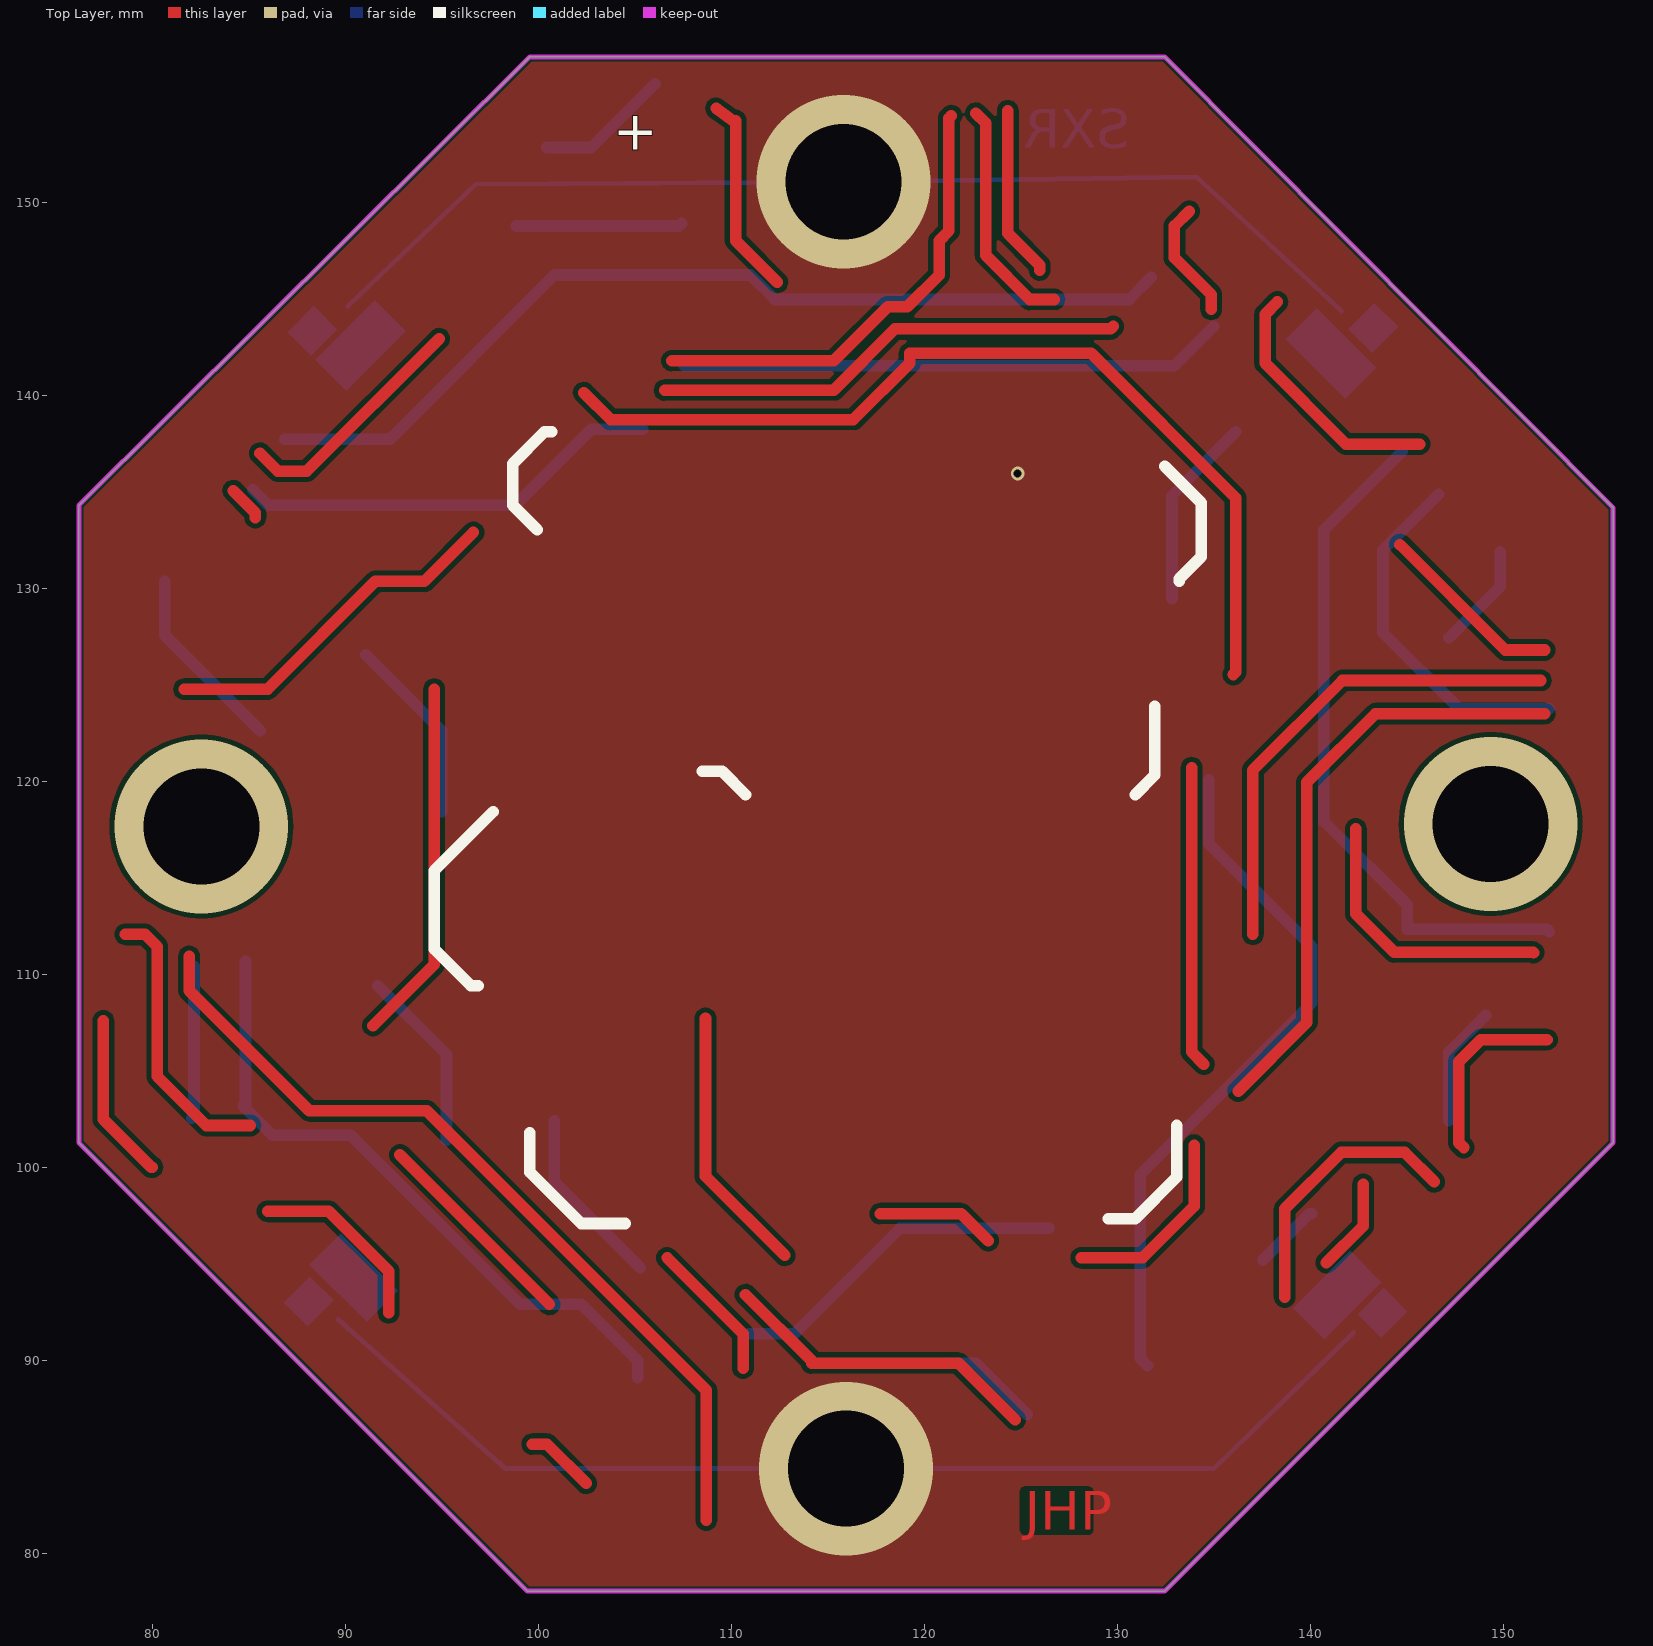
[diagram p0: Top Layer view]
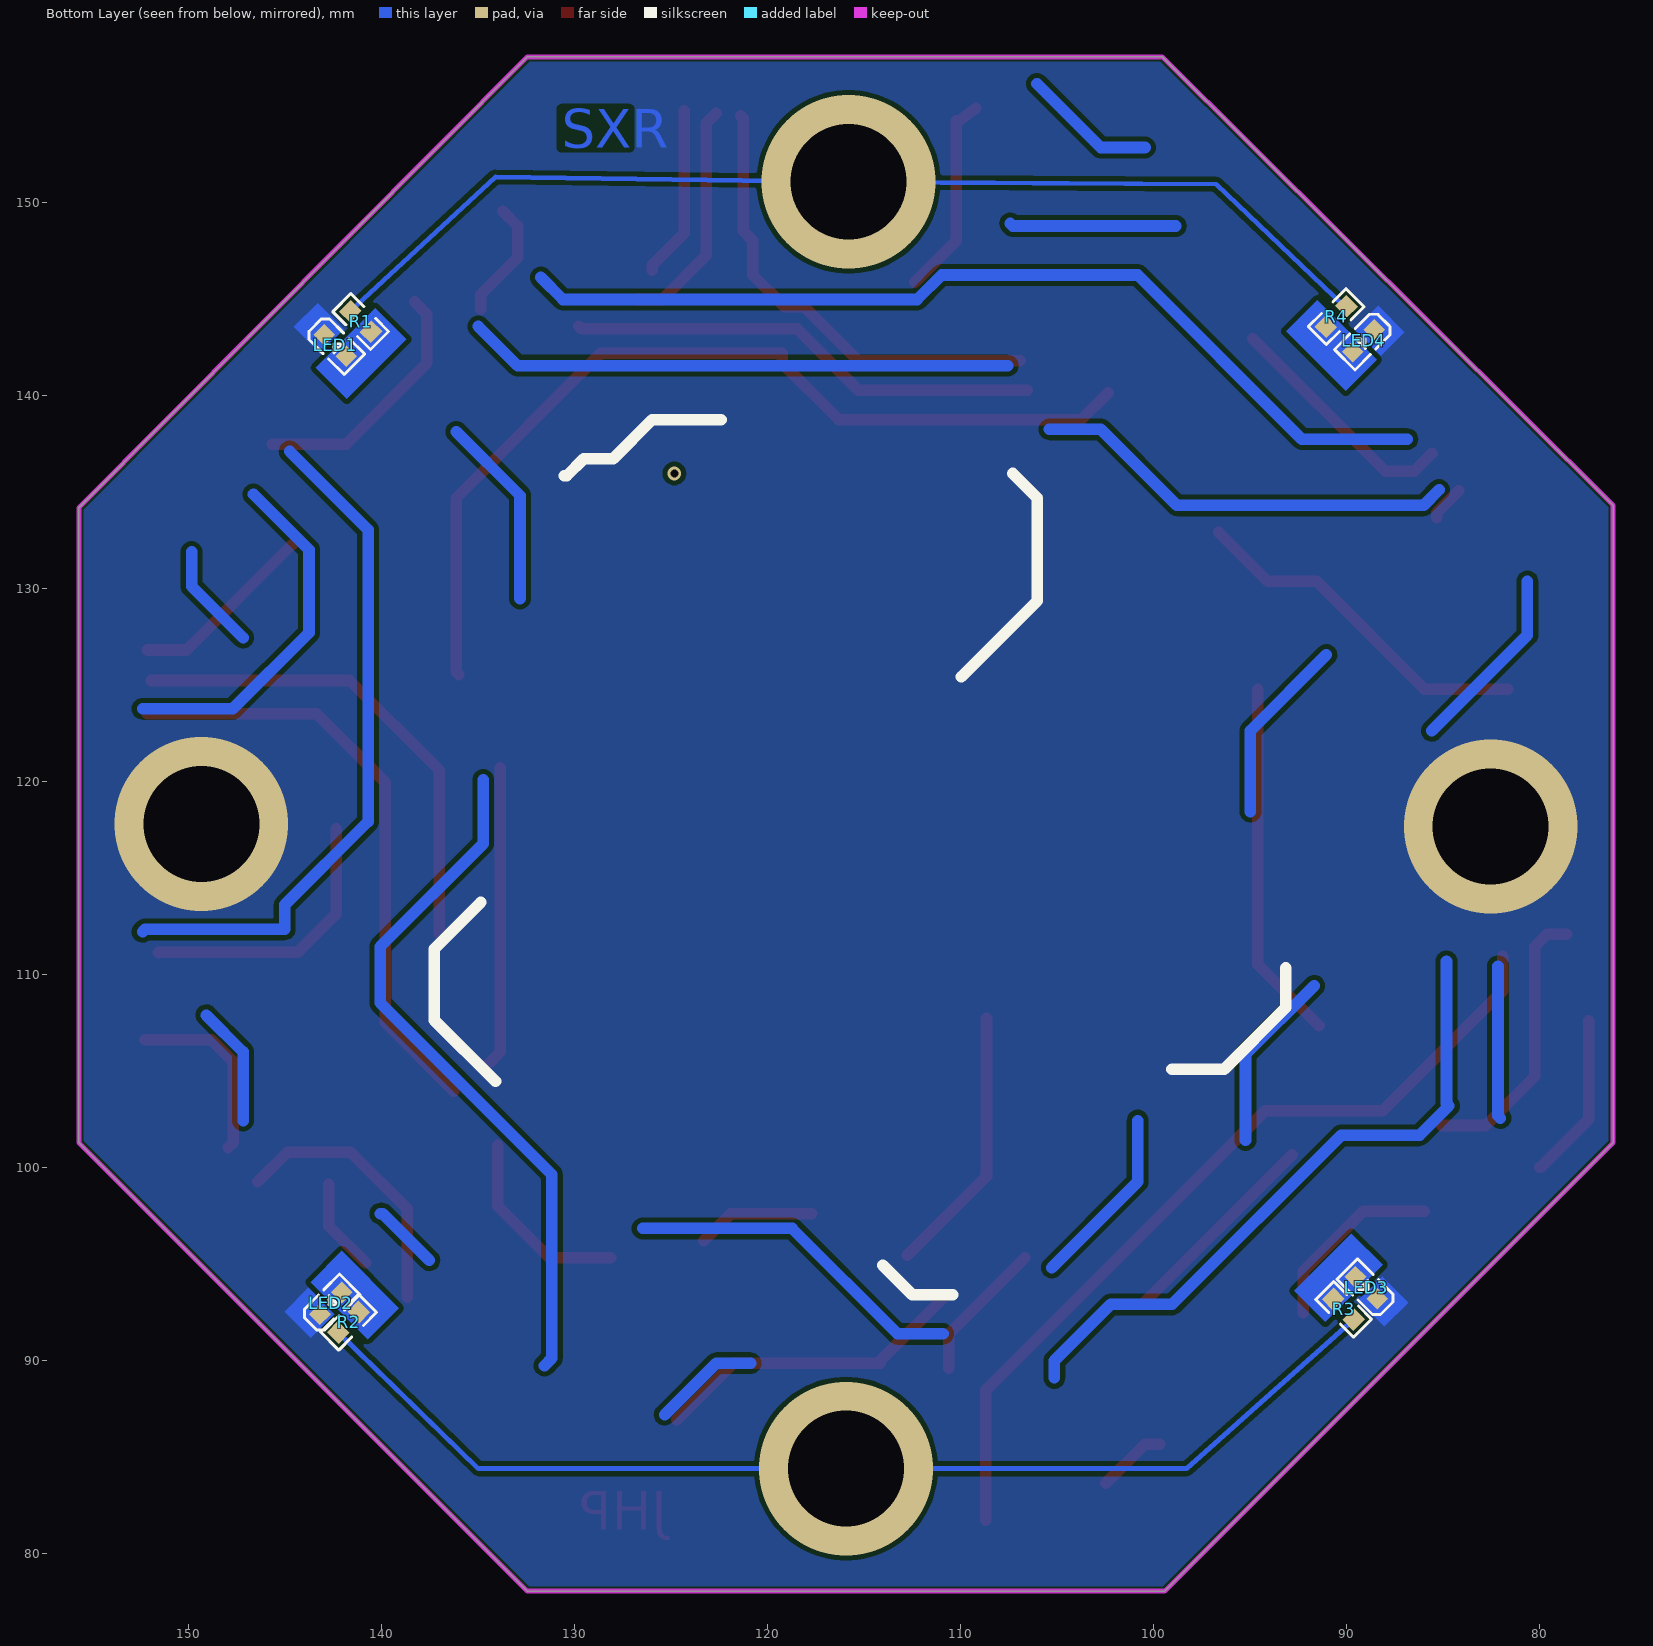
[diagram p1: Bottom Layer view, seen from below]
# Altium PCB MISC51832.pcbdoc
Units mm, origin at the board's own origin, x right, y up, seen from the top; angles counter-clockwise.
Board outline 79.5 x 79.5 mm, 2 copper layers (Top Layer, Bottom Layer), stack 1.58 mm thick; 8 components, 6 nets, 16 pads, 5 vias.

## Layer stack, top to bottom
Top Solder Mask Layer: solder mask 0.01, Dk 3.3
Top Layer: signal copper 0.035
Dielectric1: surface 1.51, FR4, Dk 4.5
Bottom Layer: signal copper 0.035
Bottom Solder Mask Layer: solder mask 0.01, Dk 3.3

## Board outline
76.2,101.265 99.441,78.024 132.461,78.024 155.702,101.265 155.702,134.158 132.461,157.526 99.568,157.526 76.2,134.285

## Design rules (kind name [scope] priority, off if disabled: settings)
BoardOutlineClearance copperThickness2oz_1 [All] p2 off: genericclearance=0.203 ignorepadtopadclearanceinfootprint=FALSE except(0: Arc-SplitContinuation Track-SplitContinuation SMDPad-SplitContinuation THPad-SplitContinuation Via-SplitContinuation Fill-SplitContinuation Region-SplitContinuation Poly-SplitContinuation Text-SplitContinuation Hole-SplitContinuation; 0.152: Arc-CutoutEdge Track-CutoutEdge SMDPad-CutoutEdge THPad-CutoutEdge Via-CutoutEdge Text-CutoutEdge; 0.175: Hole-OutlineEdge Hole-CutoutEdge; 0.254: Poly-OutlineEdge Poly-CutoutEdge; 0.3: Arc-OutlineEdge Track-OutlineEdge SMDPad-OutlineEdge THPad-OutlineEdge Via-OutlineEdge Fill-OutlineEdge Region-OutlineEdge Text-OutlineEdge Fill-CutoutEdge Region-CutoutEdge)
BoardOutlineClearance Plane_innerPlane_1 [All] p4 off: genericclearance=0.102 ignorepadtopadclearanceinfootprint=FALSE except(0: Arc-SplitContinuation Track-SplitContinuation SMDPad-SplitContinuation THPad-SplitContinuation Via-SplitContinuation Fill-SplitContinuation Region-SplitContinuation Poly-SplitContinuation Text-SplitContinuation Hole-SplitContinuation; 0.152: Arc-CutoutEdge Track-CutoutEdge SMDPad-CutoutEdge THPad-CutoutEdge Via-CutoutEdge Text-CutoutEdge; 0.175: Hole-OutlineEdge Hole-CutoutEdge; 0.254: Poly-OutlineEdge Poly-CutoutEdge; 0.3: Arc-OutlineEdge Track-OutlineEdge SMDPad-OutlineEdge THPad-OutlineEdge Via-OutlineEdge Fill-OutlineEdge Region-OutlineEdge Text-OutlineEdge Fill-CutoutEdge Region-CutoutEdge)
BoardOutlineClearance Copper_copperRegion_1 [All] p6 off: genericclearance=0.102 ignorepadtopadclearanceinfootprint=FALSE except(0: Arc-SplitContinuation Track-SplitContinuation SMDPad-SplitContinuation THPad-SplitContinuation Via-SplitContinuation Fill-SplitContinuation Region-SplitContinuation Poly-SplitContinuation Text-SplitContinuation Hole-SplitContinuation; 0.152: Arc-CutoutEdge Track-CutoutEdge SMDPad-CutoutEdge THPad-CutoutEdge Via-CutoutEdge Text-CutoutEdge; 0.175: Hole-OutlineEdge Hole-CutoutEdge; 0.254: Poly-OutlineEdge Poly-CutoutEdge; 0.3: Arc-OutlineEdge Track-OutlineEdge SMDPad-OutlineEdge THPad-OutlineEdge Via-OutlineEdge Fill-OutlineEdge Region-OutlineEdge Text-OutlineEdge Fill-CutoutEdge Region-CutoutEdge)
BoardOutlineClearance copperThickness1oz_1 [All] p8: genericclearance=0.102 ignorepadtopadclearanceinfootprint=FALSE except(0: Arc-SplitContinuation Track-SplitContinuation SMDPad-SplitContinuation THPad-SplitContinuation Via-SplitContinuation Fill-SplitContinuation Region-SplitContinuation Poly-SplitContinuation Text-SplitContinuation Hole-SplitContinuation; 0.152: Arc-CutoutEdge Track-CutoutEdge SMDPad-CutoutEdge THPad-CutoutEdge Via-CutoutEdge Text-CutoutEdge; 0.175: Hole-OutlineEdge Hole-CutoutEdge; 0.254: Poly-OutlineEdge Poly-CutoutEdge; 0.3: Arc-OutlineEdge Track-OutlineEdge SMDPad-OutlineEdge THPad-OutlineEdge Via-OutlineEdge Fill-OutlineEdge Region-OutlineEdge Text-OutlineEdge Fill-CutoutEdge Region-CutoutEdge)
Clearance copperThickness2oz [All] p1 off: gap=0.203 ignorepadtopadclearanceinfootprint=FALSE except(0.152: SMDPad-Track SMDPad-SMDPad THPad-Track SMDPad-THPad THPad-THPad Track-Via SMDPad-Via THPad-Via Via-Via Fill-SMDPad Region-SMDPad Fill-THPad Region-THPad Fill-Via Region-Via Fill-Fill Fill-Region Region-Region Arc-Track Arc-SMDPad Arc-THPad Arc-Via Fill-Arc Region-Arc Arc-Arc Text-Track SMDPad-Text Text-THPad Text-Via Fill-Text Region-Text Arc-Text Text-Text; 0.175: Hole-Track Hole-SMDPad Hole-THPad Hole-Via Fill-Hole Region-Hole Hole-Arc Hole-Text; 0.254: Poly-Track Poly-SMDPad Poly-THPad Poly-Via Poly-Fill Poly-Region Poly-Poly Poly-Arc Poly-Text Poly-Hole; 0.3: Fill-Track Region-Track)
Clearance Plane_innerPlane [All] p3 off: gap=0.102 ignorepadtopadclearanceinfootprint=FALSE except(0.152: SMDPad-Track SMDPad-SMDPad THPad-Track SMDPad-THPad THPad-THPad Track-Via SMDPad-Via THPad-Via Via-Via Fill-SMDPad Region-SMDPad Fill-THPad Region-THPad Fill-Via Region-Via Fill-Fill Fill-Region Region-Region Arc-Track Arc-SMDPad Arc-THPad Arc-Via Fill-Arc Region-Arc Arc-Arc Text-Track SMDPad-Text Text-THPad Text-Via Fill-Text Region-Text Arc-Text Text-Text; 0.175: Hole-Track Hole-SMDPad Hole-THPad Hole-Via Fill-Hole Region-Hole Hole-Arc Hole-Text; 0.254: Poly-Track Poly-SMDPad Poly-THPad Poly-Via Poly-Fill Poly-Region Poly-Poly Poly-Arc Poly-Text Poly-Hole; 0.3: Fill-Track Region-Track)
Clearance Copper_copperRegion [All] p5 off: gap=0.102 ignorepadtopadclearanceinfootprint=FALSE except(0.152: SMDPad-Track SMDPad-SMDPad THPad-Track SMDPad-THPad THPad-THPad Track-Via SMDPad-Via THPad-Via Via-Via Fill-SMDPad Region-SMDPad Fill-THPad Region-THPad Fill-Via Region-Via Fill-Fill Fill-Region Region-Region Arc-Track Arc-SMDPad Arc-THPad Arc-Via Fill-Arc Region-Arc Arc-Arc Text-Track SMDPad-Text Text-THPad Text-Via Fill-Text Region-Text Arc-Text Text-Text; 0.175: Hole-Track Hole-SMDPad Hole-THPad Hole-Via Fill-Hole Region-Hole Hole-Arc Hole-Text; 0.254: Poly-Track Poly-SMDPad Poly-THPad Poly-Via Poly-Fill Poly-Region Poly-Poly Poly-Arc Poly-Text Poly-Hole; 0.3: Fill-Track Region-Track)
Clearance copperThickness1oz [All] p7: gap=0.102 ignorepadtopadclearanceinfootprint=FALSE except(0.152: SMDPad-Track SMDPad-SMDPad THPad-Track SMDPad-THPad THPad-THPad Track-Via SMDPad-Via THPad-Via Via-Via Fill-SMDPad Region-SMDPad Fill-THPad Region-THPad Fill-Via Region-Via Fill-Fill Fill-Region Region-Region Arc-Track Arc-SMDPad Arc-THPad Arc-Via Fill-Arc Region-Arc Arc-Arc Text-Track SMDPad-Text Text-THPad Text-Via Fill-Text Region-Text Arc-Text Text-Text; 0.175: Hole-Track Hole-SMDPad Hole-THPad Hole-Via Fill-Hole Region-Hole Hole-Arc Hole-Text; 0.254: Poly-Track Poly-SMDPad Poly-THPad Poly-Via Poly-Fill Poly-Region Poly-Poly Poly-Arc Poly-Text Poly-Hole; 0.3: Fill-Track Region-Track)
DiffPairsRouting differentialPair [All] p1: maxlimit=0.152 minlimit=0.152 mostfreqgap=0.152 toplayer_minwidth=0.127 toplayer_prefwidth=0.254 toplayer_maxwidth=2.54 toplayer_mingap=0.152 toplayer_prefgap=0.152 toplayer_maxgap=0.152 bottomlayer_minwidth=0.127 bottomlayer_prefwidth=0.254 bottomlayer_maxwidth=2.54 bottomlayer_mingap=0.152 bottomlayer_prefgap=0.152 bottomlayer_maxgap=0.152 maxuncoupledlength=0.254
HoleToHoleClearance otherClearance [All] p1: gap=0.3 allowstackedmicrovias=TRUE
Length netLength [All] p1: minlimit=0 maxlimit=0
PasteMaskExpansion pasteMaskExpansion [All] p1: expansion=0
PlaneConnect innerPlane [All] p1: planeconnectstyle=Relief reliefexpansion=0.508 reliefentries=4 reliefconductorwidth=0.254 reliefairgap=0.254
PolygonConnect copperRegion [All] p1: connectstyle=Relief reliefconductorwidth=0.254 reliefentries=4 polygonreliefangle="90 Angle" airgapwidth=0.254 via.connectstyle=Relief via.reliefconductorwidth=0.254 via.reliefentries=4 via.polygonreliefangle="90 Angle" via.airgapwidth=0.254
RoutingVias viaSize [All] p1: holewidth=0.305 width=0.61 viastyle="Through Hole" minholewidth=0.3 minwidth=0.5 maxholewidth=6.3 maxwidth=10
SolderMaskExpansion solderMaskExpansion [IsVia] p1: expansion=-25.4 istentingtop=TRUE
SolderMaskExpansion solderMaskExpansion [All] p2: expansion=0.051 istentingtop=FALSE
Width copperThickness2oz_2 [All] p1 off: maxlimit=2.54 minlimit=0.203 preferedwidth=0.254
Width copperThickness1oz_2 [All] p2: maxlimit=2.54 minlimit=0.127 preferedwidth=0.254

## Components (designator, comment, footprint, x,y, rotation, side; value= is the part's Value field where it differs from the comment)
LED1 "" LED_0603 142.367,142.54 r225 bottom
LED2 "" LED_0603 142.614,92.975 r135 bottom
LED3 "" LED_0603 89.027,93.772 r45 bottom
LED4 "" LED_0603 89.165,142.776 r315 bottom
R1 "3.3k" R0603 141.097,143.81 r225 bottom
R2 "3.3k" R0603 141.725,91.959 r135 bottom
R3 "3.3k" R0603 90.17,92.629 r45 bottom
R4 "3.3k" R0603 90.551,144.064 r315 bottom

## Footprints (in the part's own frame and the unit in brackets; to place one, negate y for a bottom-side part, rotate by r counter-clockwise, add the part's x,y. Pads: shape width x height; smd on the part's side, far side on the other; paste and mask are expansions set on the pad)
LED_0603 [mil]
  rect 31.5x31.5 smd paste+0 mask+2: 1(-33.5,-0.4) 2(29.5,-0.2)
  silkscreen extent -61,-30 53,29
R0603 [mm]
  rect 0.806x0.864 smd paste-100 mask+0.051: 1(-0.753,0) 2(0.753,0)
  silkscreen extent -1.39,-0.66 1.39,0.66

## Via types
v1: diameter 9, hole 5.999, Top Layer to Bottom Layer, 4 vias
v2: diameter 0.7, hole 0.399, Top Layer to Bottom Layer, 1 vias

## Nets (pads, with @x,y where several pads share a name; then routed paths per layer and width w, separated by ;. In a path a pad name is that pad's centre, name@x,y a point inside that pad or via, vN(x,y) a via of type N, cw(c..) or ccw(c..) an arc to the next point about the centre after c; other vN are vias at no path point)
$1N377: LED1.2 R1.2
$1N381: LED2.2 R2.2
$1N385: LED3.2 R3.2
$1N390: LED4.2 R4.2
+5V: R1.1 R2.1 R3.1 R4.1 | length 450.8
  Bottom Layer w0.254: R3.1 98.298,84.374 v1(115.951,84.374) 135.001,84.374 R2.1 ; R4.1@90.145,144.597 96.774,150.922 v1(115.824,151.049) 134.112,151.303 R1.1
  Bottom Layer w0.6: 80.645,130.348 80.645,127.554 85.598,122.601 ; 82.042,102.535 82.169,102.662 82.169,110.409 ; 84.836,110.663 84.836,103.297 84.709,103.17 86.233,101.646 90.297,101.646 99.06,92.883 102.235,92.883 105.156,89.962 105.156,89.073 ; 85.222,135.086 86.024,134.285 98.806,134.285 102.743,138.222 105.41,138.222 ; 86.868,137.714 92.329,137.714 100.838,146.223 110.998,146.223 112.268,144.953 130.617,144.953 131.76,146.096 ; 91.059,126.538 94.996,122.601 94.996,118.41 ; 91.694,109.393 95.25,105.837 95.25,101.392 ; 98.859,148.761 107.313,148.761 107.442,148.89 ; 100.457,152.827 102.751,152.827 106.053,156.129 ; 100.838,102.408 100.838,99.233 105.283,94.788 ; 107.569,141.524 132.969,141.524 135.001,143.556 ; 110.924,91.359 113.284,91.359 118.745,96.82 126.492,96.82 ; 120.896,89.835 122.682,89.835 125.349,87.168 ; 131.572,89.708 131.191,90.089 131.191,99.614 140.081,108.504 140.081,111.425 134.747,116.759 134.747,120.061 ; 132.842,129.459 132.842,134.793 136.144,138.095 ; 137.541,95.169 139.954,97.582 140.081,97.582 ; 144.78,137.079 140.716,133.015 140.716,117.902 145.034,113.584 145.034,112.314 152.273,112.314 152.4,112.187 ; 146.649,134.859 143.776,131.986 143.776,127.688 147.72,123.744 152.4,123.744 ; 147.193,102.408 147.193,105.964 149.098,107.869 ; 147.193,127.427 149.86,130.094 149.86,131.872
  other v2: 124.841,135.936
GND: LED1.1 LED2.1 LED3.1 LED4.1 | length 470.4
  Top Layer w0.6: 77.47,107.576 77.47,102.476 79.951,99.995 80.01,99.995 ; 78.613,112.06 79.629,112.06 80.264,111.425 80.264,104.694 82.804,102.154 85.09,102.154 ; 81.661,124.76 85.979,124.76 91.567,130.348 94.107,130.348 96.647,132.888 ; 81.915,110.917 81.915,109.139 88.138,102.916 94.234,102.916 108.712,88.438 108.712,81.707 ; 84.201,135.047 85.344,133.904 85.344,133.65 ; 85.586,136.988 86.512,136.063 88.011,136.063 94.869,142.921 ; 85.979,97.709 89.154,97.709 92.254,94.609 92.254,92.443 ; 91.444,107.325 94.615,110.496 94.615,124.76 ; 92.837,100.63 100.584,92.883 ; 99.695,85.644 100.457,85.644 102.489,83.612 ; 102.362,140.127 103.759,138.73 116.332,138.73 119.253,141.651 119.253,142.159 128.651,142.159 136.144,134.666 136.144,125.649 136.017,125.522 ; 106.553,140.254 115.316,140.254 118.491,143.429 129.667,143.429 129.794,143.556 ; 106.68,95.296 110.617,91.359 110.617,89.581 ; 106.934,141.778 115.316,141.778 118.11,144.572 119.126,144.572 120.777,146.223 120.777,148.001 121.285,148.509 121.285,154.351 121.412,154.478 ; 108.673,107.704 108.673,99.526 112.776,95.423 ; 109.22,154.859 110.211,154.148 110.236,154.224 110.236,148.001 112.395,145.842 ; 110.744,93.391 114.173,89.962 114.173,89.835 121.793,89.835 124.714,86.914 ; 117.729,97.582 121.92,97.582 123.317,96.185 ; 122.682,154.605 123.19,154.097 123.19,147.239 125.476,144.953 126.746,144.953 ; 124.333,154.732 124.333,148.382 125.984,146.731 125.984,146.477 ; 128.143,95.296 131.318,95.296 133.985,97.963 133.985,101.138 ; 133.731,149.525 132.969,148.763 132.969,147.112 134.874,145.207 134.874,144.445 ; 133.858,120.696 133.858,105.964 134.493,105.329 ; 136.271,103.932 139.827,107.488 139.827,119.934 143.383,123.49 152.146,123.49 ; 137.033,112.06 137.033,120.569 141.673,125.209 151.951,125.209 ; 138.303,144.826 137.668,144.191 137.668,141.651 141.859,137.46 145.669,137.46 ; 138.684,93.264 138.684,97.836 141.605,100.757 144.907,100.757 146.431,99.233 ; 140.843,95.042 142.748,96.947 142.748,99.106 ; 142.367,117.521 142.367,113.127 144.362,111.132 151.554,111.132 151.574,111.112 ; 144.653,132.253 150.114,126.792 152.146,126.792 ; 147.955,101.011 147.701,101.265 147.701,105.456 148.844,106.599 152.273,106.599
  other v1: 82.55,117.648 149.352,117.775

## Polygon pours and split planes (outlines as drawn)
+5V on Top Layer (solid, remove dead copper, pour order 0): 99.568,157.526 132.461,157.526 155.702,134.158 155.702,101.265 132.461,78.024 99.441,78.024 76.2,101.265 76.2,134.285
GND on Bottom Layer (solid, remove dead copper, pour order 2): 99.379,157.338 132.334,157.272 155.702,134.158 155.702,101.265 132.461,78.024 99.441,78.024 76.2,101.265 76.2,134.285

## Keep-outs
Board Outline Layer:
  the board outline again, w0.254

## Other copper
Top Layer:
  text "JHP" at 125.222,81.199 h2
Bottom Layer:
  region net $1N381: 139.129,92.692 140.736,91.085 143.695,94.043 142.087,95.651
  region net $1N390: 88.453,141.823 90.061,140.215 93.146,143.3 91.539,144.908
  region net $1N377: 141.814,139.807 143.422,141.415 140.337,144.5 138.729,142.893
  region net GND: 87.024,143.267 88.251,142.039 89.601,143.388 88.373,144.616
  region net GND: 141.981,143.414 143.208,142.186 144.558,143.535 143.33,144.763
  region net GND: 142.462,92.385 143.689,91.157 145.039,92.506 143.811,93.734
  region net GND: 86.824,92.975 88.052,91.747 89.401,93.096 88.173,94.324
  region net $1N385: 91.11,91.98 92.718,93.588 89.759,96.546 88.151,94.938
  text "SXR" at 130.683,152.827 h2

## Silkscreen, mask and mechanical layers (free items; w line width, h text height)
Top Silkscreen Layer:
  lines w0.6: 96.901,109.393 96.517,109.393 94.615,111.295 94.615,115.362 97.663,118.41 ; 99.568,101.773 99.568,99.741 102.235,97.074 104.521,97.074 ; 99.949,133.015 98.679,134.285 98.679,136.444 100.33,138.095 100.711,138.095 ; 108.502,120.505 109.537,120.505 110.744,119.299 ; 129.54,97.328 130.938,97.328 133.096,99.486 133.096,102.154 ; 130.937,119.299 131.953,120.315 131.953,123.871 ; 132.461,136.317 134.366,134.412 134.366,131.618 133.223,130.475 133.223,130.348
  text "+" at 103.886,152.7 h2
Bottom Silkscreen Layer:
  lines w0.6: 93.168,110.315 93.168,108.265 96.358,105.075 99.06,105.075 ; 107.315,135.936 106.045,134.666 106.045,129.332 109.982,125.395 ; 110.414,93.391 112.522,93.391 114.046,94.915 ; 122.428,138.73 125.984,138.73 128.016,136.698 129.54,136.698 130.429,135.809 130.556,135.809 ; 134.112,104.44 137.287,107.615 137.287,111.298 134.874,113.711
Top Solder Mask Layer:
  drawing of 175 lines, arcs and shapes, not listed
Bottom Solder Mask Layer:
  drawing of 118 lines, arcs and shapes, not listed
  text "2025" at 105.537,125.395 h6
  text "巳" at 103.124,119.426 h8
  text "已" at 133.985,118.918 h8